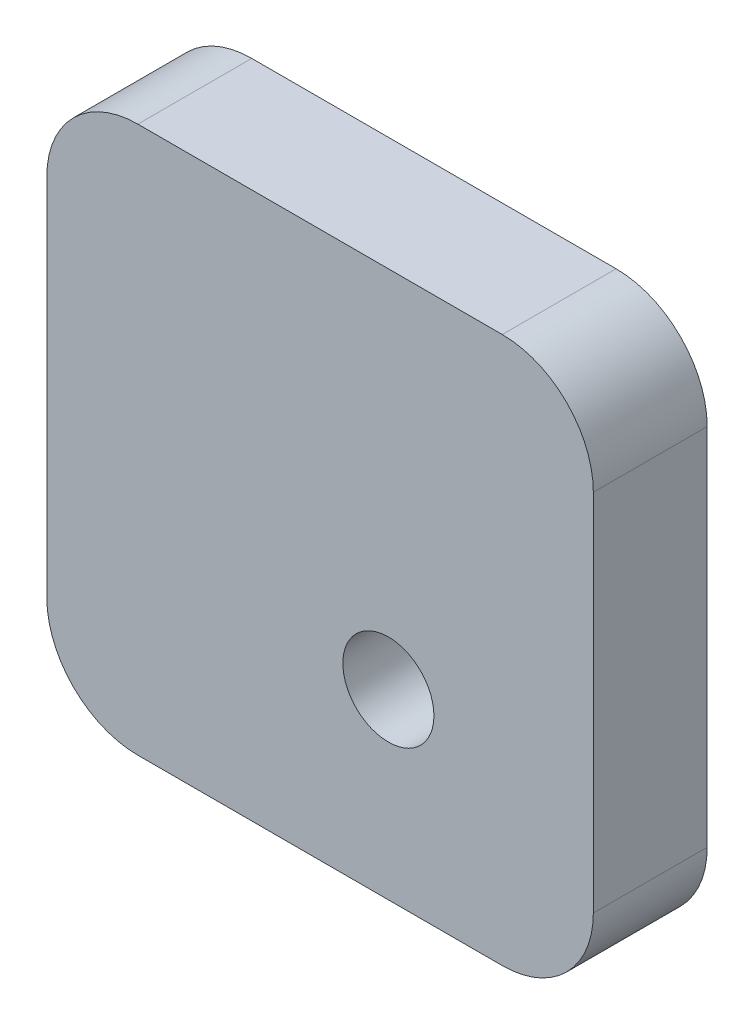
SolidWorks part; units mm, degrees
material "钢板25/Q235A"
ref_plane "Front Plane" through (0, 0, 0) normal (0, 0, 1) x (1, 0, 0)
ref_plane "Top Plane" through (0, 0, 0) normal (0, 1, 0) x (1, 0, 0)
ref_plane "Right Plane" through (0, 0, 0) normal (1, 0, 0) x (0, 0, -1)
sketch "Sketch1" plane through (0, 0, 0) normal (0, 0, 1) x (1, 0, 0)
  line L1 (0, 0) -> (120, 0)
  line L2 (0, 0) -> (0, 120)
  line L3 (0, 120) -> (120, 120)
  line L4 (120, 0) -> (120, 120)
  circle A0 centre (75, 40) radius 10
  dimension "D3" = 20
  dimension "D1" = 120
  dimension "D2" = 120
  dimension "D4" = 40
  dimension "D5" = 45
extrude "Boss-Extrude1" add sketch "Sketch1" along normal blind 25
fillet "Fillet1" radius 20 4 edges at (0, 0, 12.5) (120, 0, 12.5) (120, 120, 12.5) (0, 120, 12.5)
